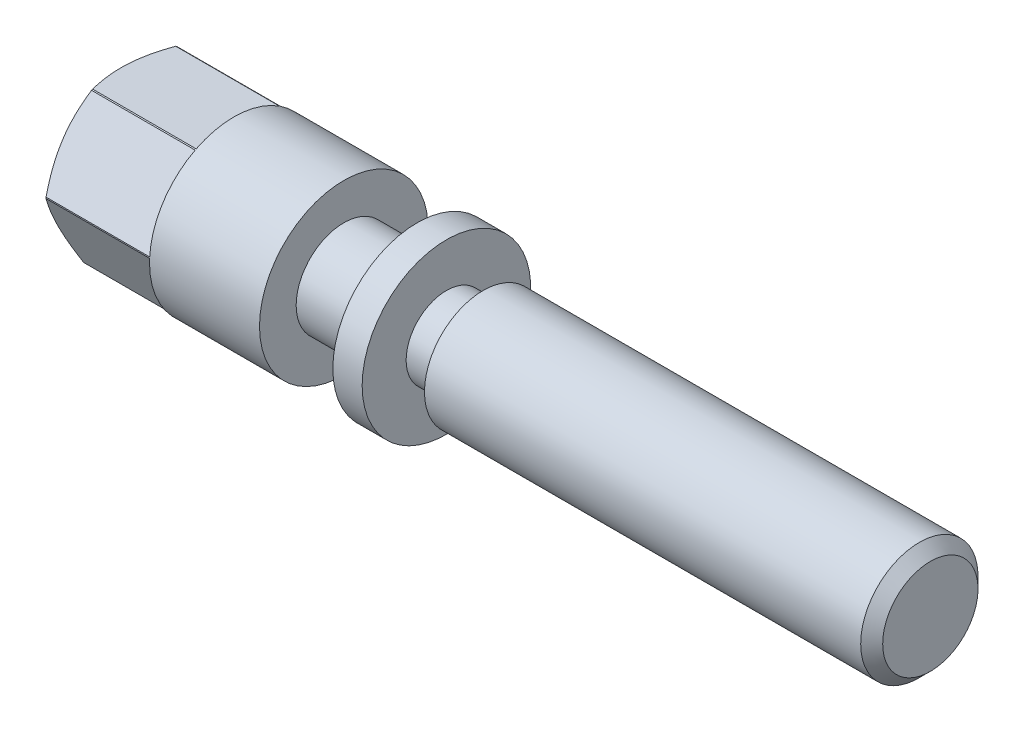
SolidWorks part; units mm, degrees
ref_plane "Front Plane" through (0, 0, 0) normal (0, 0, 1) x (1, 0, 0)
ref_plane "Top Plane" through (0, 0, 0) normal (0, 1, 0) x (1, 0, 0)
ref_plane "Right Plane" through (0, 0, 0) normal (1, 0, 0) x (0, 0, -1)
sketch "Sketch1" plane through (0, 0, 0) normal (0, 0, 1) x (1, 0, 0)
  line L0 (0, 0) -> (110, 0) construction
  line L1 (0, 0) -> (0, 10)
  line L2 (0.866, 11.5) -> (30, 11.5)
  line L3 (30, 11.5) -> (30, 6.5)
  line L4 (30, 6.5) -> (40, 6.5)
  line L5 (40, 6.5) -> (40, 11.5)
  line L6 (40, 11.5) -> (44, 11.5)
  line L7 (44, 11.5) -> (44, 5.5)
  line L8 (44, 5.5) -> (49, 5.5)
  line L9 (49, 5.5) -> (49, 8)
  line L10 (49, 8) -> (110, 8)
  line L11 (110, 8) -> (110, 0)
  line L12 (0, 0) -> (110, 0)
  line L13 (0, 10) -> (0.866, 11.5)
  dimension "D1" = 110
  dimension "D2" = 8
  dimension "D3" = 5.5
  dimension "D4" = 6.5
  dimension "D5" = 11.5
  dimension "D6" = 11.5
  dimension "D7" = 66
  dimension "D8" = 5
  dimension "D9" = 10
  dimension "D10" = 40
  dimension "D11" = 30
  dimension "D12" = 10
revolve "Revolve1" add sketch "Sketch1" angle 360 about L0
cosmetic thread "Cosmetic Thread1" parameters "D2"=13.835
hole_wizard "M12 Tapped Hole1" positions "3DSketch2" profile "Sketch3" tap size "M12" standard "GB"
sketch3d "3DSketch2"
  point P0 (0, 0, 0)
  dimension "D1" = 0
sketch "Sketch3" plane through (0, 0, 0) normal (0, 1, 0) x (0, 0, 1)
  line L0 (0, 0) -> (0, 26.3144)
  line L1 (0, 26.3144) -> (5.1, 23.25)
  line L2 (5.1, 23.25) -> (5.1, 0.925)
  line L3 (5.1, 0.925) -> (6.025, 0)
  line L5 (6.025, 0) -> (0, 0)
  line L6 (-5.1, 0.925) -> (-6.025, 0) construction
  line L10 (0, 26.3144) -> (-5.1, 23.25) construction
  line L11 (0, -6.35) -> (0, 107.95) construction
  dimension "螺纹孔钻头直径" = 10.2
  dimension "螺纹孔钻头深度" = 23.25
  dimension "近端锥形沉头孔直径" = 12.05
  dimension "近端锥形沉头孔角度" = 90
  dimension "导头角度" = 118
cosmetic thread "Hole thread 1" parameters "D1"=18, "D2"=12
sketch "Sketch4" plane through (0, 0, 0) normal (-1, 0, 0) x (0, 0, 1)
  line L1 (5.2274, 10.296) -> (-6.3029, 9.675)
  line L2 (-6.3029, 9.675) -> (-11.5303, -0.621)
  line L3 (-11.5303, -0.621) -> (-5.2274, -10.296)
  line L4 (-5.2274, -10.296) -> (6.3029, -9.675)
  line L5 (6.3029, -9.675) -> (11.5303, 0.621)
  line L6 (11.5303, 0.621) -> (5.2274, 10.296)
  circle A0 centre (0, 0) radius 10 construction
  circle A1 centre (0, 0) radius 21.575
  dimension "D1" = 20
extrude "Cut-Extrude1" cut sketch "Sketch4" against normal blind 15
chamfer "Chamfer1" distance 1.5 angle 45 1 edges at (110, 0, 8)
